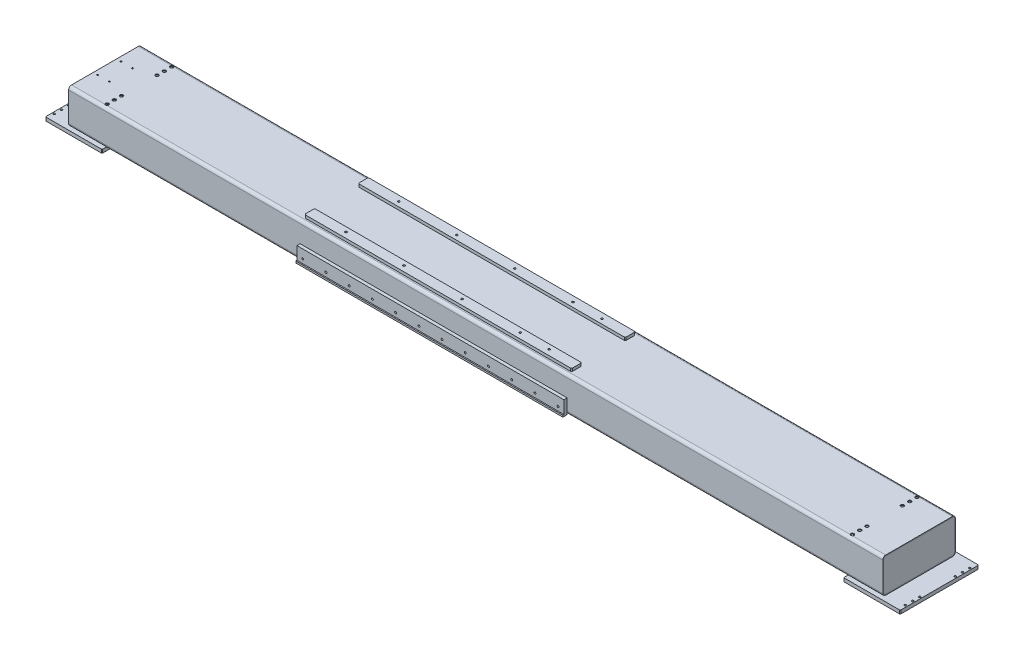
from build123d import *

# Parameters (mm, degrees)
F_250_X_120_X_3_0_1_DEPTH      = 2805
EXTRUDE_1_DEPTH                = 5
EXTRUDE_2_DEPTH                = 12
EXTRUDE_2_2_DEPTH              = 12
SKETCH_9_W                     = 920
SKETCH_9_H                     = 35
EXTRUDE_3_DEPTH                = 10
EXTRUDE_3_2_DEPTH              = 10
HOLE_WIZARD_M8_1_AT_2_COUNT    = 2
HOLE_WIZARD_M8_1_AT_2_PITCH    = 182
HOLE_WIZARD_M8_1_AT_3_COUNT    = 2
HOLE_WIZARD_M8_1_AT_3_PITCH    = 200
HOLE_WIZARD_M8_1_AT_4_COUNT    = 2
HOLE_WIZARD_M8_1_AT_4_PITCH    = 270.414496653
HOLE_WIZARD_M8_1_AT_5_COUNT    = 2
HOLE_WIZARD_M8_1_AT_5_PITCH    = 400
HOLE_WIZARD_M8_1_AT_6_COUNT    = 2
HOLE_WIZARD_M8_1_AT_6_PITCH    = 439.458758019
HOLE_WIZARD_M8_1_AT_7_COUNT    = 2
HOLE_WIZARD_M8_1_AT_7_PITCH    = 600
HOLE_WIZARD_M8_1_AT_8_COUNT    = 2
HOLE_WIZARD_M8_1_AT_8_PITCH    = 626.996012746
HOLE_WIZARD_M8_1_AT_9_COUNT    = 2
HOLE_WIZARD_M8_1_AT_9_PITCH    = 723.273115773
HOLE_WIZARD_M8_1_AT_10_COUNT   = 2
HOLE_WIZARD_M8_1_AT_10_PITCH   = 700
SKETCH_12_W                    = 920
SKETCH_12_H                    = 50
EXTRUDE_4_DEPTH                = 15
HOLE_WIZARD_M6_1_AT_2_COUNT    = 2
HOLE_WIZARD_M6_1_AT_2_PITCH    = 450
HOLE_WIZARD_M6_1_AT_3_COUNT    = 2
HOLE_WIZARD_M6_1_AT_3_PITCH    = 900
HOLE_WIZARD_M6_2_AT_2_COUNT    = 2
HOLE_WIZARD_M6_2_AT_2_PITCH    = 80
HOLE_WIZARD_M6_2_AT_3_COUNT    = 2
HOLE_WIZARD_M6_2_AT_3_PITCH    = 40
HOLE_WIZARD_M6_2_AT_4_COUNT    = 2
HOLE_WIZARD_M6_2_AT_4_PITCH    = 89.4427191
CHAMFER_1_SIZE                 = 3
CHAMFER_2_SIZE                 = 3
SKETCH_22_W                    = 3.3
SKETCH_22_H                    = 12
HOLE_WIZARD_M6_1_2_AT_2_COUNT  = 2
HOLE_WIZARD_M6_1_2_AT_2_PITCH  = 182
HOLE_WIZARD_M6_1_2_AT_3_COUNT  = 2
HOLE_WIZARD_M6_1_2_AT_3_PITCH  = 219.10727966
HOLE_WIZARD_M6_1_2_AT_4_COUNT  = 2
HOLE_WIZARD_M6_1_2_AT_4_PITCH  = 122
HOLE_WIZARD_M6_1_2_AT_5_COUNT  = 2
HOLE_WIZARD_M6_1_2_AT_5_PITCH  = 147
HOLE_WIZARD_M6_1_2_AT_6_COUNT  = 2
HOLE_WIZARD_M6_1_2_AT_6_PITCH  = 172
HOLE_WIZARD_M6_1_2_AT_7_COUNT  = 2
HOLE_WIZARD_M6_1_2_AT_7_PITCH  = 250.415654463
HOLE_WIZARD_M6_1_2_AT_8_COUNT  = 2
HOLE_WIZARD_M6_1_2_AT_8_PITCH  = 233.950849539
HOLE_WIZARD_M6_1_2_AT_9_COUNT  = 2
HOLE_WIZARD_M6_1_2_AT_9_PITCH  = 183.709009033
HOLE_WIZARD_M6_1_2_AT_10_COUNT = 2
HOLE_WIZARD_M6_1_2_AT_10_PITCH = 188.743211798
HOLE_WIZARD_M6_1_2_AT_11_COUNT = 2
HOLE_WIZARD_M6_1_2_AT_11_PITCH = 50
HOLE_WIZARD_M6_1_2_AT_12_COUNT = 2
HOLE_WIZARD_M6_1_2_AT_12_PITCH = 25
HOLE_WIZARD_M6_1_2_AT_13_COUNT = 2
HOLE_WIZARD_M6_1_2_AT_13_PITCH = 2932.1065806
HOLE_WIZARD_M6_1_2_AT_14_COUNT = 2
HOLE_WIZARD_M6_1_2_AT_14_PITCH = 2932.426299159
HOLE_WIZARD_M6_1_2_AT_15_COUNT = 2
HOLE_WIZARD_M6_1_2_AT_15_PITCH = 2750.454507895
HOLE_WIZARD_M6_1_2_AT_16_COUNT = 2
HOLE_WIZARD_M6_1_2_AT_16_PITCH = 2750.113634016
HOLE_WIZARD_M6_1_2_AT_17_COUNT = 2
HOLE_WIZARD_M6_1_2_AT_17_PITCH = 2750
HOLE_WIZARD_M6_1_2_AT_18_COUNT = 2
HOLE_WIZARD_M6_1_2_AT_18_PITCH = 2932
HOLE_WIZARD_M6_1_2_AT_19_COUNT = 2
HOLE_WIZARD_M6_1_2_AT_19_PITCH = 2753.926106489
HOLE_WIZARD_M6_1_2_AT_20_COUNT = 2
HOLE_WIZARD_M6_1_2_AT_20_PITCH = 2755.373658871
HOLE_WIZARD_M6_1_2_AT_21_COUNT = 2
HOLE_WIZARD_M6_1_2_AT_21_PITCH = 2937.040687495
HOLE_WIZARD_M6_1_2_AT_22_COUNT = 2
HOLE_WIZARD_M6_1_2_AT_22_PITCH = 2935.682714464
HOLE_WIZARD_M6_1_2_AT_23_COUNT = 2
HOLE_WIZARD_M6_1_2_AT_23_PITCH = 2934.537101486
HOLE_WIZARD_M6_1_2_AT_24_COUNT = 2
HOLE_WIZARD_M6_1_2_AT_24_PITCH = 2752.704851596
HOLE_WIZARD_1_AT_2_COUNT       = 2
HOLE_WIZARD_1_AT_2_PITCH       = 2568
HOLE_WIZARD_1_AT_3_COUNT       = 2
HOLE_WIZARD_1_AT_3_PITCH       = 2570.896341745
HOLE_WIZARD_1_AT_4_COUNT       = 2
HOLE_WIZARD_1_AT_4_PITCH       = 2568.121687148
HOLE_WIZARD_1_AT_5_COUNT       = 2
HOLE_WIZARD_1_AT_5_PITCH       = 2568.486714001
HOLE_WIZARD_1_AT_6_COUNT       = 2
HOLE_WIZARD_1_AT_6_PITCH       = 2572.203918821
HOLE_WIZARD_1_AT_7_COUNT       = 2
HOLE_WIZARD_1_AT_7_PITCH       = 2573.753678968
HOLE_WIZARD_1_AT_8_COUNT       = 2
HOLE_WIZARD_1_AT_8_PITCH       = 172
HOLE_WIZARD_1_AT_9_COUNT       = 2
HOLE_WIZARD_1_AT_9_PITCH       = 147
HOLE_WIZARD_1_AT_10_COUNT      = 2
HOLE_WIZARD_1_AT_10_PITCH      = 50
HOLE_WIZARD_1_AT_11_COUNT      = 2
HOLE_WIZARD_1_AT_11_PITCH      = 25
HOLE_WIZARD_1_AT_12_COUNT      = 2
HOLE_WIZARD_1_AT_12_PITCH      = 122
SKETCH_26_W                    = 920
SKETCH_26_H                    = 44
CUT_EXTRUDE_1_DEPTH            = 4
HOLE_WIZARD_M8_2_AT_2_COUNT    = 2
HOLE_WIZARD_M8_2_AT_2_PITCH    = 80
HOLE_WIZARD_M8_2_AT_3_COUNT    = 2
HOLE_WIZARD_M8_2_AT_3_PITCH    = 160
HOLE_WIZARD_M8_2_AT_4_COUNT    = 2
HOLE_WIZARD_M8_2_AT_4_PITCH    = 240
HOLE_WIZARD_M8_2_AT_5_COUNT    = 2
HOLE_WIZARD_M8_2_AT_5_PITCH    = 320
HOLE_WIZARD_M8_2_AT_6_COUNT    = 2
HOLE_WIZARD_M8_2_AT_6_PITCH    = 400
HOLE_WIZARD_M8_2_AT_7_COUNT    = 2
HOLE_WIZARD_M8_2_AT_7_PITCH    = 480
HOLE_WIZARD_M8_2_AT_8_COUNT    = 2
HOLE_WIZARD_M8_2_AT_8_PITCH    = 560
HOLE_WIZARD_M8_2_AT_9_COUNT    = 2
HOLE_WIZARD_M8_2_AT_9_PITCH    = 640
HOLE_WIZARD_M8_2_AT_10_COUNT   = 2
HOLE_WIZARD_M8_2_AT_10_PITCH   = 720
HOLE_WIZARD_M8_2_AT_11_COUNT   = 2
HOLE_WIZARD_M8_2_AT_11_PITCH   = 800
HOLE_WIZARD_M8_2_AT_12_COUNT   = 2
HOLE_WIZARD_M8_2_AT_12_PITCH   = 880


with BuildPart() as part:
    # Sketch11 → 矩型管 250 X 120 X 3.0(1) (new body)
    with BuildSketch(Plane.YZ.offset(-1402.5)):
        with BuildLine():
            Line((-50, -125), (50, -125))
            ThreePointArc((50, -125), (57.071067812, -122.071067812), (60, -115))
            Line((60, -115), (60, 115))
            ThreePointArc((60, 115), (57.071067812, 122.071067812), (50, 125))
            Line((50, 125), (-50, 125))
            ThreePointArc((-50, 125), (-57.071067812, 122.071067812), (-60, 115))
            Line((-60, 115), (-60, -115))
            ThreePointArc((-60, -115), (-57.071067812, -122.071067812), (-50, -125))
        make_face()
        with BuildLine():
            Line((-50, -122), (50, -122))
            ThreePointArc((50, -122), (54.949747468, -119.949747468), (57, -115))
            Line((57, -115), (57, 115))
            ThreePointArc((57, 115), (54.949747468, 119.949747468), (50, 122))
            Line((50, 122), (-50, 122))
            ThreePointArc((-50, 122), (-54.949747468, 119.949747468), (-57, 115))
            Line((-57, 115), (-57, -115))
            ThreePointArc((-57, -115), (-54.949747468, -119.949747468), (-50, -122))
        make_face(mode=Mode.SUBTRACT)
    extrude(amount=F_250_X_120_X_3_0_1_DEPTH)


with BuildPart() as body_2:
    # 草图3 → 凸台-拉伸1 (new body)
    with BuildSketch(Plane.ZY.offset(1402.5)):
        with BuildLine():
            Line((-122, -50), (-122, 50))
            ThreePointArc((-122, 50), (-119.949747468, 54.949747468), (-115, 57))
            Line((-115, 57), (115, 57))
            ThreePointArc((115, 57), (119.949747468, 54.949747468), (122, 50))
            Line((122, 50), (122, -50))
            ThreePointArc((122, -50), (119.949747468, -54.949747468), (115, -57))
            Line((115, -57), (-115, -57))
            ThreePointArc((-115, -57), (-119.949747468, -54.949747468), (-122, -50))
        make_face()
    extrude(amount=-EXTRUDE_1_DEPTH)


with BuildPart() as body_3:
    # 镜向1: mirrored copy
    add(body_2.part.mirror(Plane.XY))


with BuildPart() as body_4:
    # 镜向2: mirrored copy
    add(body_2.part.mirror(Plane(origin=(0, 0, 0), x_dir=(0, 0, 1), z_dir=(1, 0, 0))))


with BuildPart() as body_5:
    # Mirror 2 2: mirrored copy
    add(body_3.part.mirror(Plane(origin=(0, 0, 0), x_dir=(0, 0, 1), z_dir=(1, 0, 0))))


with BuildPart() as body_6:
    # 草图5 → 凸台-拉伸2 (new body)
    with BuildSketch(Plane(origin=(0, -60, -185), x_dir=(1, 0, 0), z_dir=(0, -1, 0))):
        Polygon((-1470.5, 320), (-1279.5, 320), (-1277.5, 318), (-1277.5, 52), (-1279.5, 50), (-1470.5, 50), (-1472.5, 52), (-1472.5, 318), align=None)
    extrude(amount=EXTRUDE_2_DEPTH)

    # 草图22 → Hole Wizard M6 _1 2 (revolve, cut)
    with BuildSketch(Plane(origin=(-1466, -60, -61), x_dir=(0, 0, 1), z_dir=(1, 0, 0))):
        with Locations((1.65, 6)):
            Rectangle(SKETCH_22_W, SKETCH_22_H)
    hole_wizard_m6_1_2 = revolve(axis=Axis((-1466, -53.65, -61), (0, -1, 0)), mode=Mode.SUBTRACT)

    # Hole Wizard M6 _1 2 at 2: Hole Wizard M6 _1 2 ×2
    with Locations(*[(i * HOLE_WIZARD_M6_1_2_AT_2_PITCH, 0, 0) for i in range(1, HOLE_WIZARD_M6_1_2_AT_2_COUNT)]):
        add(hole_wizard_m6_1_2, mode=Mode.SUBTRACT)

    # Hole Wizard M6 _1 2 at 3: Hole Wizard M6 _1 2 ×2
    with Locations(*[Vector(0.8306433281560934, -1.9052030489669335e-15, 0.5568048683244143) * (i * HOLE_WIZARD_M6_1_2_AT_3_PITCH) for i in range(1, HOLE_WIZARD_M6_1_2_AT_3_COUNT)]):
        add(hole_wizard_m6_1_2, mode=Mode.SUBTRACT)

    # Hole Wizard M6 _1 2 at 4: Hole Wizard M6 _1 2 ×2
    with Locations(*[(0, 0, i * HOLE_WIZARD_M6_1_2_AT_4_PITCH) for i in range(1, HOLE_WIZARD_M6_1_2_AT_4_COUNT)]):
        add(hole_wizard_m6_1_2, mode=Mode.SUBTRACT)

    # Hole Wizard M6 _1 2 at 5: Hole Wizard M6 _1 2 ×2
    with Locations(*[(0, 0, i * HOLE_WIZARD_M6_1_2_AT_5_PITCH) for i in range(1, HOLE_WIZARD_M6_1_2_AT_5_COUNT)]):
        add(hole_wizard_m6_1_2, mode=Mode.SUBTRACT)

    # Hole Wizard M6 _1 2 at 6: Hole Wizard M6 _1 2 ×2
    with Locations(*[(0, 0, i * HOLE_WIZARD_M6_1_2_AT_6_PITCH) for i in range(1, HOLE_WIZARD_M6_1_2_AT_6_COUNT)]):
        add(hole_wizard_m6_1_2, mode=Mode.SUBTRACT)

    # Hole Wizard M6 _1 2 at 7: Hole Wizard M6 _1 2 ×2
    with Locations(*[Vector(0.7267916232732317, -2.3479926408873147e-15, 0.6868580175988783) * (i * HOLE_WIZARD_M6_1_2_AT_7_PITCH) for i in range(1, HOLE_WIZARD_M6_1_2_AT_7_COUNT)]):
        add(hole_wizard_m6_1_2, mode=Mode.SUBTRACT)

    # Hole Wizard M6 _1 2 at 8: Hole Wizard M6 _1 2 ×2
    with Locations(*[Vector(0.7779411802037216, -2.1487803380109524e-15, 0.6283371070876212) * (i * HOLE_WIZARD_M6_1_2_AT_8_PITCH) for i in range(1, HOLE_WIZARD_M6_1_2_AT_8_COUNT)]):
        add(hole_wizard_m6_1_2, mode=Mode.SUBTRACT)

    # Hole Wizard M6 _1 2 at 9: Hole Wizard M6 _1 2 ×2
    with Locations(*[Vector(0.9906971952965136, 0, -0.1360847795736969) * (i * HOLE_WIZARD_M6_1_2_AT_9_PITCH) for i in range(1, HOLE_WIZARD_M6_1_2_AT_9_COUNT)]):
        add(hole_wizard_m6_1_2, mode=Mode.SUBTRACT)

    # Hole Wizard M6 _1 2 at 10: Hole Wizard M6 _1 2 ×2
    with Locations(*[Vector(0.9642730896957256, 0, -0.2649101894768476) * (i * HOLE_WIZARD_M6_1_2_AT_10_PITCH) for i in range(1, HOLE_WIZARD_M6_1_2_AT_10_COUNT)]):
        add(hole_wizard_m6_1_2, mode=Mode.SUBTRACT)

    # Hole Wizard M6 _1 2 at 11: Hole Wizard M6 _1 2 ×2
    with Locations(*[(0, 0, -i * HOLE_WIZARD_M6_1_2_AT_11_PITCH) for i in range(1, HOLE_WIZARD_M6_1_2_AT_11_COUNT)]):
        add(hole_wizard_m6_1_2, mode=Mode.SUBTRACT)

    # Hole Wizard M6 _1 2 at 12: Hole Wizard M6 _1 2 ×2
    with Locations(*[(0, 0, -i * HOLE_WIZARD_M6_1_2_AT_12_PITCH) for i in range(1, HOLE_WIZARD_M6_1_2_AT_12_COUNT)]):
        add(hole_wizard_m6_1_2, mode=Mode.SUBTRACT)


with BuildPart() as body_7:
    # 草图5 → Extrude 2 2 (new body)
    with BuildSketch(Plane(origin=(0, -60, -185), x_dir=(1, 0, 0), z_dir=(0, -1, 0))):
        Polygon((1472.5, 318), (1470.5, 320), (1279.5, 320), (1277.5, 318), (1277.5, 52), (1279.5, 50), (1470.5, 50), (1472.5, 52), align=None)
    extrude(amount=EXTRUDE_2_2_DEPTH)

    # Hole Wizard M6 _1 2 at 13: Hole Wizard M6 _1 2 ×2
    with Locations(*[Vector(0.9999636505026536, 0, -0.008526293063631086) * (i * HOLE_WIZARD_M6_1_2_AT_13_PITCH) for i in range(1, HOLE_WIZARD_M6_1_2_AT_13_COUNT)]):
        add(hole_wizard_m6_1_2, mode=Mode.SUBTRACT)

    # Hole Wizard M6 _1 2 at 14: Hole Wizard M6 _1 2 ×2
    with Locations(*[Vector(0.9998546257891517, 0, -0.01705072690636343) * (i * HOLE_WIZARD_M6_1_2_AT_14_PITCH) for i in range(1, HOLE_WIZARD_M6_1_2_AT_14_COUNT)]):
        add(hole_wizard_m6_1_2, mode=Mode.SUBTRACT)

    # Hole Wizard M6 _1 2 at 15: Hole Wizard M6 _1 2 ×2
    with Locations(*[Vector(0.9998347517133228, 0, -0.018178813667514955) * (i * HOLE_WIZARD_M6_1_2_AT_15_PITCH) for i in range(1, HOLE_WIZARD_M6_1_2_AT_15_COUNT)]):
        add(hole_wizard_m6_1_2, mode=Mode.SUBTRACT)

    # Hole Wizard M6 _1 2 at 16: Hole Wizard M6 _1 2 ×2
    with Locations(*[Vector(0.9999586802470746, 0, -0.009090533456791589) * (i * HOLE_WIZARD_M6_1_2_AT_16_PITCH) for i in range(1, HOLE_WIZARD_M6_1_2_AT_16_COUNT)]):
        add(hole_wizard_m6_1_2, mode=Mode.SUBTRACT)

    # Hole Wizard M6 _1 2 at 17: Hole Wizard M6 _1 2 ×2
    with Locations(*[(i * HOLE_WIZARD_M6_1_2_AT_17_PITCH, 0, 0) for i in range(1, HOLE_WIZARD_M6_1_2_AT_17_COUNT)]):
        add(hole_wizard_m6_1_2, mode=Mode.SUBTRACT)

    # Hole Wizard M6 _1 2 at 18: Hole Wizard M6 _1 2 ×2
    with Locations(*[(i * HOLE_WIZARD_M6_1_2_AT_18_PITCH, 0, 0) for i in range(1, HOLE_WIZARD_M6_1_2_AT_18_COUNT)]):
        add(hole_wizard_m6_1_2, mode=Mode.SUBTRACT)

    # Hole Wizard M6 _1 2 at 19: Hole Wizard M6 _1 2 ×2
    with Locations(*[Vector(0.9985743602635353, 0, 0.05337833853045079) * (i * HOLE_WIZARD_M6_1_2_AT_19_PITCH) for i in range(1, HOLE_WIZARD_M6_1_2_AT_19_COUNT)]):
        add(hole_wizard_m6_1_2, mode=Mode.SUBTRACT)

    # Hole Wizard M6 _1 2 at 20: Hole Wizard M6 _1 2 ×2
    with Locations(*[Vector(0.9980497531238023, 0, 0.062423475468106907) * (i * HOLE_WIZARD_M6_1_2_AT_20_PITCH) for i in range(1, HOLE_WIZARD_M6_1_2_AT_20_COUNT)]):
        add(hole_wizard_m6_1_2, mode=Mode.SUBTRACT)

    # Hole Wizard M6 _1 2 at 21: Hole Wizard M6 _1 2 ×2
    with Locations(*[Vector(0.9982837529230445, 0, 0.05856234839794122) * (i * HOLE_WIZARD_M6_1_2_AT_21_PITCH) for i in range(1, HOLE_WIZARD_M6_1_2_AT_21_COUNT)]):
        add(hole_wizard_m6_1_2, mode=Mode.SUBTRACT)

    # Hole Wizard M6 _1 2 at 22: Hole Wizard M6 _1 2 ×2
    with Locations(*[Vector(0.9987455338939073, 0, 0.05007353120136575) * (i * HOLE_WIZARD_M6_1_2_AT_22_PITCH) for i in range(1, HOLE_WIZARD_M6_1_2_AT_22_COUNT)]):
        add(hole_wizard_m6_1_2, mode=Mode.SUBTRACT)

    # Hole Wizard M6 _1 2 at 23: Hole Wizard M6 _1 2 ×2
    with Locations(*[Vector(0.9991354338355168, 0, 0.04157384820188713) * (i * HOLE_WIZARD_M6_1_2_AT_23_PITCH) for i in range(1, HOLE_WIZARD_M6_1_2_AT_23_COUNT)]):
        add(hole_wizard_m6_1_2, mode=Mode.SUBTRACT)

    # Hole Wizard M6 _1 2 at 24: Hole Wizard M6 _1 2 ×2
    with Locations(*[Vector(0.9990173840851833, 0, 0.04432004394850631) * (i * HOLE_WIZARD_M6_1_2_AT_24_PITCH) for i in range(1, HOLE_WIZARD_M6_1_2_AT_24_COUNT)]):
        add(hole_wizard_m6_1_2, mode=Mode.SUBTRACT)


with BuildPart() as body_8:
    # 草图9 → 凸台-拉伸3 (new body)
    with BuildSketch(Plane(origin=(0, 60, 0), x_dir=(1, 0, 0), z_dir=(0, 1, 0))):
        with Locations((-145, 92.5)):
            Rectangle(SKETCH_9_W, SKETCH_9_H)
    extrude(amount=EXTRUDE_3_DEPTH)


with BuildPart() as body_9:
    # 草图9 → Extrude 3 2 (new body)
    with BuildSketch(Plane(origin=(0, 60, 0), x_dir=(1, 0, 0), z_dir=(0, 1, 0))):
        with Locations((-145, -92.5)):
            Rectangle(SKETCH_9_W, SKETCH_9_H)
    extrude(amount=EXTRUDE_3_2_DEPTH)


with BuildPart() as hole_wizard_m8_1_tool:
    # 草图11 → Hole Wizard M8 _1 (revolve)
    with BuildSketch(Plane(origin=(-481, 70, -91), x_dir=(0, 0, 1), z_dir=(1, 0, 0))):
        Polygon((0, 0), (0, 21.792926105), (3.4, 19.75), (3.4, 0), align=None)
    hole_wizard_m8_1 = revolve(axis=Axis((-481, 76.35, -91), (0, -1, 0)))


with BuildPart() as part_1:
    add(part.part)

    # Hole Wizard M8 _1: cut by hole_wizard_m8_1_tool
    add(hole_wizard_m8_1_tool.part, mode=Mode.SUBTRACT)


with BuildPart() as body_8_1:
    add(body_8.part)

    # Hole Wizard M8 _1: cut by hole_wizard_m8_1_tool
    add(hole_wizard_m8_1_tool.part, mode=Mode.SUBTRACT)


with BuildPart() as hole_wizard_m8_1_at_2_tool:
    # Hole Wizard M8 _1 at 2: Hole Wizard M8 _1 ×2
    with Locations(*[(0, 0, i * HOLE_WIZARD_M8_1_AT_2_PITCH) for i in range(1, HOLE_WIZARD_M8_1_AT_2_COUNT)]):
        add(hole_wizard_m8_1)


with BuildPart() as part_2:
    add(part_1.part)

    # Hole Wizard M8 _1 at 2: cut by hole_wizard_m8_1_at_2_tool
    add(hole_wizard_m8_1_at_2_tool.part, mode=Mode.SUBTRACT)


with BuildPart() as body_9_1:
    add(body_9.part)

    # Hole Wizard M8 _1 at 2: cut by hole_wizard_m8_1_at_2_tool
    add(hole_wizard_m8_1_at_2_tool.part, mode=Mode.SUBTRACT)


with BuildPart() as hole_wizard_m8_1_at_3_tool:
    # Hole Wizard M8 _1 at 3: Hole Wizard M8 _1 ×2
    with Locations(*[(i * HOLE_WIZARD_M8_1_AT_3_PITCH, 0, 0) for i in range(1, HOLE_WIZARD_M8_1_AT_3_COUNT)]):
        add(hole_wizard_m8_1)


with BuildPart() as part_3:
    add(part_2.part)

    # Hole Wizard M8 _1 at 3: cut by hole_wizard_m8_1_at_3_tool
    add(hole_wizard_m8_1_at_3_tool.part, mode=Mode.SUBTRACT)


with BuildPart() as body_8_2:
    add(body_8_1.part)

    # Hole Wizard M8 _1 at 3: cut by hole_wizard_m8_1_at_3_tool
    add(hole_wizard_m8_1_at_3_tool.part, mode=Mode.SUBTRACT)


with BuildPart() as hole_wizard_m8_1_at_4_tool:
    # Hole Wizard M8 _1 at 4: Hole Wizard M8 _1 ×2
    with Locations(*[Vector(0.7396053187813598, 0, 0.6730408400909437) * (i * HOLE_WIZARD_M8_1_AT_4_PITCH) for i in range(1, HOLE_WIZARD_M8_1_AT_4_COUNT)]):
        add(hole_wizard_m8_1)


with BuildPart() as part_4:
    add(part_3.part)

    # Hole Wizard M8 _1 at 4: cut by hole_wizard_m8_1_at_4_tool
    add(hole_wizard_m8_1_at_4_tool.part, mode=Mode.SUBTRACT)


with BuildPart() as body_9_2:
    add(body_9_1.part)

    # Hole Wizard M8 _1 at 4: cut by hole_wizard_m8_1_at_4_tool
    add(hole_wizard_m8_1_at_4_tool.part, mode=Mode.SUBTRACT)


with BuildPart() as hole_wizard_m8_1_at_5_tool:
    # Hole Wizard M8 _1 at 5: Hole Wizard M8 _1 ×2
    with Locations(*[(i * HOLE_WIZARD_M8_1_AT_5_PITCH, 0, 0) for i in range(1, HOLE_WIZARD_M8_1_AT_5_COUNT)]):
        add(hole_wizard_m8_1)


with BuildPart() as part_5:
    add(part_4.part)

    # Hole Wizard M8 _1 at 5: cut by hole_wizard_m8_1_at_5_tool
    add(hole_wizard_m8_1_at_5_tool.part, mode=Mode.SUBTRACT)


with BuildPart() as body_8_3:
    add(body_8_2.part)

    # Hole Wizard M8 _1 at 5: cut by hole_wizard_m8_1_at_5_tool
    add(hole_wizard_m8_1_at_5_tool.part, mode=Mode.SUBTRACT)


with BuildPart() as hole_wizard_m8_1_at_6_tool:
    # Hole Wizard M8 _1 at 6: Hole Wizard M8 _1 ×2
    with Locations(*[Vector(0.9102105549169733, 0, 0.4141458024871621) * (i * HOLE_WIZARD_M8_1_AT_6_PITCH) for i in range(1, HOLE_WIZARD_M8_1_AT_6_COUNT)]):
        add(hole_wizard_m8_1)


with BuildPart() as part_6:
    add(part_5.part)

    # Hole Wizard M8 _1 at 6: cut by hole_wizard_m8_1_at_6_tool
    add(hole_wizard_m8_1_at_6_tool.part, mode=Mode.SUBTRACT)


with BuildPart() as body_9_3:
    add(body_9_2.part)

    # Hole Wizard M8 _1 at 6: cut by hole_wizard_m8_1_at_6_tool
    add(hole_wizard_m8_1_at_6_tool.part, mode=Mode.SUBTRACT)


with BuildPart() as hole_wizard_m8_1_at_7_tool:
    # Hole Wizard M8 _1 at 7: Hole Wizard M8 _1 ×2
    with Locations(*[(i * HOLE_WIZARD_M8_1_AT_7_PITCH, 0, 0) for i in range(1, HOLE_WIZARD_M8_1_AT_7_COUNT)]):
        add(hole_wizard_m8_1)


with BuildPart() as part_7:
    add(part_6.part)

    # Hole Wizard M8 _1 at 7: cut by hole_wizard_m8_1_at_7_tool
    add(hole_wizard_m8_1_at_7_tool.part, mode=Mode.SUBTRACT)


with BuildPart() as body_8_4:
    add(body_8_3.part)

    # Hole Wizard M8 _1 at 7: cut by hole_wizard_m8_1_at_7_tool
    add(hole_wizard_m8_1_at_7_tool.part, mode=Mode.SUBTRACT)


with BuildPart() as hole_wizard_m8_1_at_8_tool:
    # Hole Wizard M8 _1 at 8: Hole Wizard M8 _1 ×2
    with Locations(*[Vector(0.9569438844942066, 0, 0.2902729782965312) * (i * HOLE_WIZARD_M8_1_AT_8_PITCH) for i in range(1, HOLE_WIZARD_M8_1_AT_8_COUNT)]):
        add(hole_wizard_m8_1)


with BuildPart() as part_8:
    add(part_7.part)

    # Hole Wizard M8 _1 at 8: cut by hole_wizard_m8_1_at_8_tool
    add(hole_wizard_m8_1_at_8_tool.part, mode=Mode.SUBTRACT)


with BuildPart() as body_9_4:
    add(body_9_3.part)

    # Hole Wizard M8 _1 at 8: cut by hole_wizard_m8_1_at_8_tool
    add(hole_wizard_m8_1_at_8_tool.part, mode=Mode.SUBTRACT)


with BuildPart() as hole_wizard_m8_1_at_9_tool:
    # Hole Wizard M8 _1 at 9: Hole Wizard M8 _1 ×2
    with Locations(*[Vector(0.9678225067882815, 0, 0.2516338517649143) * (i * HOLE_WIZARD_M8_1_AT_9_PITCH) for i in range(1, HOLE_WIZARD_M8_1_AT_9_COUNT)]):
        add(hole_wizard_m8_1)


with BuildPart() as part_9:
    add(part_8.part)

    # Hole Wizard M8 _1 at 9: cut by hole_wizard_m8_1_at_9_tool
    add(hole_wizard_m8_1_at_9_tool.part, mode=Mode.SUBTRACT)


with BuildPart() as body_9_5:
    add(body_9_4.part)

    # Hole Wizard M8 _1 at 9: cut by hole_wizard_m8_1_at_9_tool
    add(hole_wizard_m8_1_at_9_tool.part, mode=Mode.SUBTRACT)

    # 倒角2
    chamfer_2_edges = [body_9_5.edges().sort_by_distance(p)[0] for p in [
        (-605, 65, 110),
        (-605, 65, 75),
        (315, 65, 75),
        (315, 65, 110),
    ]]
    chamfer(chamfer_2_edges, length=CHAMFER_2_SIZE)


with BuildPart() as hole_wizard_m8_1_at_10_tool:
    # Hole Wizard M8 _1 at 10: Hole Wizard M8 _1 ×2
    with Locations(*[(i * HOLE_WIZARD_M8_1_AT_10_PITCH, 0, 0) for i in range(1, HOLE_WIZARD_M8_1_AT_10_COUNT)]):
        add(hole_wizard_m8_1)


with BuildPart() as part_10:
    add(part_9.part)

    # Hole Wizard M8 _1 at 10: cut by hole_wizard_m8_1_at_10_tool
    add(hole_wizard_m8_1_at_10_tool.part, mode=Mode.SUBTRACT)

    # 草图18 → Hole Wizard M6 _1 (revolve, cut)
    with BuildSketch(Plane(origin=(305, -15, -125), x_dir=(0, 1, 0), z_dir=(1, 0, 0))):
        Polygon((0, 0), (0, 16.502151548), (2.5, 15), (2.5, 0), align=None)
    hole_wizard_m6_1 = revolve(axis=Axis((305, -15, -131.35), (0, 0, 1)), mode=Mode.SUBTRACT)

    # Hole Wizard M6 _1 at 2: Hole Wizard M6 _1 ×2
    with Locations(*[(-i * HOLE_WIZARD_M6_1_AT_2_PITCH, 0, 0) for i in range(1, HOLE_WIZARD_M6_1_AT_2_COUNT)]):
        add(hole_wizard_m6_1, mode=Mode.SUBTRACT)

    # Hole Wizard M6 _1 at 3: Hole Wizard M6 _1 ×2
    with Locations(*[(-i * HOLE_WIZARD_M6_1_AT_3_PITCH, 0, 0) for i in range(1, HOLE_WIZARD_M6_1_AT_3_COUNT)]):
        add(hole_wizard_m6_1, mode=Mode.SUBTRACT)

    # 草图20 → M6 螺纹孔2 (revolve, cut)
    with BuildSketch(Plane(origin=(-1387.5, 60, 40), x_dir=(0, 0, 1), z_dir=(1, 0, 0))):
        Polygon((0, 0), (0, 16.502151548), (2.5, 15), (2.5, 0), align=None)
    hole_wizard_m6_2 = revolve(axis=Axis((-1387.5, 66.35, 40), (0, -1, 0)), mode=Mode.SUBTRACT)

    # M6 螺纹孔2 at 2: M6 螺纹孔2 ×2
    with Locations(*[(0, 0, -i * HOLE_WIZARD_M6_2_AT_2_PITCH) for i in range(1, HOLE_WIZARD_M6_2_AT_2_COUNT)]):
        add(hole_wizard_m6_2, mode=Mode.SUBTRACT)

    # M6 螺纹孔2 at 3: M6 螺纹孔2 ×2
    with Locations(*[(i * HOLE_WIZARD_M6_2_AT_3_PITCH, 0, 0) for i in range(1, HOLE_WIZARD_M6_2_AT_3_COUNT)]):
        add(hole_wizard_m6_2, mode=Mode.SUBTRACT)

    # M6 螺纹孔2 at 4: M6 螺纹孔2 ×2
    with Locations(*[Vector(0.447213595499958, 3.1180628964785753e-15, -0.894427190999916) * (i * HOLE_WIZARD_M6_2_AT_4_PITCH) for i in range(1, HOLE_WIZARD_M6_2_AT_4_COUNT)]):
        add(hole_wizard_m6_2, mode=Mode.SUBTRACT)

    # 草图25 → 打孔尺寸(%根据)内六角圆柱头螺钉的类型1 (revolve, cut)
    with BuildSketch(Plane(origin=(1284, 60, 61), x_dir=(0, 0, 1), z_dir=(1, 0, 0))):
        Polygon((0, 0), (0, 132), (3.3, 132), (3.3, 6.8), (5.5, 6.8), (5.5, 0), align=None)
    hole_wizard_1 = revolve(axis=Axis((1284, 66.35, 61), (0, -1, 0)), mode=Mode.SUBTRACT)

    # 打孔尺寸(%根据)内六角圆柱头螺钉的类型1 at 2: 打孔尺寸(%根据)内六角圆柱头螺钉的类型1 ×2
    with Locations(*[(-i * HOLE_WIZARD_1_AT_2_PITCH, 0, 0) for i in range(1, HOLE_WIZARD_1_AT_2_COUNT)]):
        add(hole_wizard_1, mode=Mode.SUBTRACT)

    # 打孔尺寸(%根据)内六角圆柱头螺钉的类型1 at 3: 打孔尺寸(%根据)内六角圆柱头螺钉的类型1 ×2
    with Locations(*[Vector(-0.9988734116975495, 0, -0.04745426644357505) * (i * HOLE_WIZARD_1_AT_3_PITCH) for i in range(1, HOLE_WIZARD_1_AT_3_COUNT)]):
        add(hole_wizard_1, mode=Mode.SUBTRACT)

    # 打孔尺寸(%根据)内六角圆柱头螺钉的类型1 at 4: 打孔尺寸(%根据)内六角圆柱头螺钉的类型1 ×2
    with Locations(*[Vector(-0.9999526162842554, 0, 0.009734741202144355) * (i * HOLE_WIZARD_1_AT_4_PITCH) for i in range(1, HOLE_WIZARD_1_AT_4_COUNT)]):
        add(hole_wizard_1, mode=Mode.SUBTRACT)

    # 打孔尺寸(%根据)内六角圆柱头螺钉的类型1 at 5: 打孔尺寸(%根据)内六角圆柱头螺钉的类型1 ×2
    with Locations(*[Vector(-0.9998105055407085, 0, 0.019466715450559086) * (i * HOLE_WIZARD_1_AT_5_PITCH) for i in range(1, HOLE_WIZARD_1_AT_5_COUNT)]):
        add(hole_wizard_1, mode=Mode.SUBTRACT)

    # 打孔尺寸(%根据)内六角圆柱头螺钉的类型1 at 6: 打孔尺寸(%根据)内六角圆柱头螺钉的类型1 ×2
    with Locations(*[Vector(-0.9983656354806839, 0, -0.05714943474130069) * (i * HOLE_WIZARD_1_AT_6_PITCH) for i in range(1, HOLE_WIZARD_1_AT_6_COUNT)]):
        add(hole_wizard_1, mode=Mode.SUBTRACT)

    # 打孔尺寸(%根据)内六角圆柱头螺钉的类型1 at 7: 打孔尺寸(%根据)内六角圆柱头螺钉的类型1 ×2
    with Locations(*[Vector(-0.99776447955577, 0, -0.06682846202632091) * (i * HOLE_WIZARD_1_AT_7_PITCH) for i in range(1, HOLE_WIZARD_1_AT_7_COUNT)]):
        add(hole_wizard_1, mode=Mode.SUBTRACT)

    # 打孔尺寸(%根据)内六角圆柱头螺钉的类型1 at 8: 打孔尺寸(%根据)内六角圆柱头螺钉的类型1 ×2
    with Locations(*[(0, 0, -i * HOLE_WIZARD_1_AT_8_PITCH) for i in range(1, HOLE_WIZARD_1_AT_8_COUNT)]):
        add(hole_wizard_1, mode=Mode.SUBTRACT)

    # 打孔尺寸(%根据)内六角圆柱头螺钉的类型1 at 9: 打孔尺寸(%根据)内六角圆柱头螺钉的类型1 ×2
    with Locations(*[(0, 0, -i * HOLE_WIZARD_1_AT_9_PITCH) for i in range(1, HOLE_WIZARD_1_AT_9_COUNT)]):
        add(hole_wizard_1, mode=Mode.SUBTRACT)

    # 打孔尺寸(%根据)内六角圆柱头螺钉的类型1 at 10: 打孔尺寸(%根据)内六角圆柱头螺钉的类型1 ×2
    with Locations(*[(0, 0, i * HOLE_WIZARD_1_AT_10_PITCH) for i in range(1, HOLE_WIZARD_1_AT_10_COUNT)]):
        add(hole_wizard_1, mode=Mode.SUBTRACT)

    # 打孔尺寸(%根据)内六角圆柱头螺钉的类型1 at 11: 打孔尺寸(%根据)内六角圆柱头螺钉的类型1 ×2
    with Locations(*[(0, 0, i * HOLE_WIZARD_1_AT_11_PITCH) for i in range(1, HOLE_WIZARD_1_AT_11_COUNT)]):
        add(hole_wizard_1, mode=Mode.SUBTRACT)

    # 打孔尺寸(%根据)内六角圆柱头螺钉的类型1 at 12: 打孔尺寸(%根据)内六角圆柱头螺钉的类型1 ×2
    with Locations(*[(0, 0, -i * HOLE_WIZARD_1_AT_12_PITCH) for i in range(1, HOLE_WIZARD_1_AT_12_COUNT)]):
        add(hole_wizard_1, mode=Mode.SUBTRACT)


with BuildPart() as body_8_5:
    add(body_8_4.part)

    # Hole Wizard M8 _1 at 10: cut by hole_wizard_m8_1_at_10_tool
    add(hole_wizard_m8_1_at_10_tool.part, mode=Mode.SUBTRACT)

    # 倒角1
    chamfer_1_edges = [body_8_5.edges().sort_by_distance(p)[0] for p in [
        (-605, 65, -110),
        (315, 65, -110),
        (315, 65, -75),
        (-605, 65, -75),
    ]]
    chamfer(chamfer_1_edges, length=CHAMFER_1_SIZE)


with BuildPart() as body_10:
    # 草图12 → 凸台-拉伸4 (new body)
    with BuildSketch(Plane(origin=(0, 65, 125), x_dir=(1, 0, 0), z_dir=(0, 0, -1))):
        with Locations((-145, 100)):
            Rectangle(SKETCH_12_W, SKETCH_12_H)
    extrude(amount=-EXTRUDE_4_DEPTH)

    # 草图26 → 切除-拉伸1 (cut)
    with BuildSketch(Plane.XY.offset(140)):
        with Locations((-145, -32)):
            Rectangle(SKETCH_26_W, SKETCH_26_H)
    extrude(amount=-CUT_EXTRUDE_1_DEPTH, mode=Mode.SUBTRACT)


with BuildPart() as hole_wizard_m8_2_tool:
    # 草图14 → M8 螺纹孔2 (revolve)
    with BuildSketch(Plane(origin=(-585, -40, 136), x_dir=(0, -1, 0), z_dir=(1, 0, 0))):
        Polygon((0, 0), (0, 21.792926105), (3.4, 19.75), (3.4, 0), align=None)
    hole_wizard_m8_2 = revolve(axis=Axis((-585, -40, 142.35), (0, 0, -1)))


with BuildPart() as part_11:
    add(part_10.part)

    # M8 螺纹孔2: cut by hole_wizard_m8_2_tool
    add(hole_wizard_m8_2_tool.part, mode=Mode.SUBTRACT)


with BuildPart() as body_10_1:
    add(body_10.part)

    # M8 螺纹孔2: cut by hole_wizard_m8_2_tool
    add(hole_wizard_m8_2_tool.part, mode=Mode.SUBTRACT)


with BuildPart() as hole_wizard_m8_2_at_2_tool:
    # M8 螺纹孔2 at 2: M8 螺纹孔2 ×2
    with Locations(*[(i * HOLE_WIZARD_M8_2_AT_2_PITCH, 0, 0) for i in range(1, HOLE_WIZARD_M8_2_AT_2_COUNT)]):
        add(hole_wizard_m8_2)


with BuildPart() as part_12:
    add(part_11.part)

    # M8 螺纹孔2 at 2: cut by hole_wizard_m8_2_at_2_tool
    add(hole_wizard_m8_2_at_2_tool.part, mode=Mode.SUBTRACT)


with BuildPart() as body_10_2:
    add(body_10_1.part)

    # M8 螺纹孔2 at 2: cut by hole_wizard_m8_2_at_2_tool
    add(hole_wizard_m8_2_at_2_tool.part, mode=Mode.SUBTRACT)


with BuildPart() as hole_wizard_m8_2_at_3_tool:
    # M8 螺纹孔2 at 3: M8 螺纹孔2 ×2
    with Locations(*[(i * HOLE_WIZARD_M8_2_AT_3_PITCH, 0, 0) for i in range(1, HOLE_WIZARD_M8_2_AT_3_COUNT)]):
        add(hole_wizard_m8_2)


with BuildPart() as part_13:
    add(part_12.part)

    # M8 螺纹孔2 at 3: cut by hole_wizard_m8_2_at_3_tool
    add(hole_wizard_m8_2_at_3_tool.part, mode=Mode.SUBTRACT)


with BuildPart() as body_10_3:
    add(body_10_2.part)

    # M8 螺纹孔2 at 3: cut by hole_wizard_m8_2_at_3_tool
    add(hole_wizard_m8_2_at_3_tool.part, mode=Mode.SUBTRACT)


with BuildPart() as hole_wizard_m8_2_at_4_tool:
    # M8 螺纹孔2 at 4: M8 螺纹孔2 ×2
    with Locations(*[(i * HOLE_WIZARD_M8_2_AT_4_PITCH, 0, 0) for i in range(1, HOLE_WIZARD_M8_2_AT_4_COUNT)]):
        add(hole_wizard_m8_2)


with BuildPart() as part_14:
    add(part_13.part)

    # M8 螺纹孔2 at 4: cut by hole_wizard_m8_2_at_4_tool
    add(hole_wizard_m8_2_at_4_tool.part, mode=Mode.SUBTRACT)


with BuildPart() as body_10_4:
    add(body_10_3.part)

    # M8 螺纹孔2 at 4: cut by hole_wizard_m8_2_at_4_tool
    add(hole_wizard_m8_2_at_4_tool.part, mode=Mode.SUBTRACT)


with BuildPart() as hole_wizard_m8_2_at_5_tool:
    # M8 螺纹孔2 at 5: M8 螺纹孔2 ×2
    with Locations(*[(i * HOLE_WIZARD_M8_2_AT_5_PITCH, 0, 0) for i in range(1, HOLE_WIZARD_M8_2_AT_5_COUNT)]):
        add(hole_wizard_m8_2)


with BuildPart() as part_15:
    add(part_14.part)

    # M8 螺纹孔2 at 5: cut by hole_wizard_m8_2_at_5_tool
    add(hole_wizard_m8_2_at_5_tool.part, mode=Mode.SUBTRACT)


with BuildPart() as body_10_5:
    add(body_10_4.part)

    # M8 螺纹孔2 at 5: cut by hole_wizard_m8_2_at_5_tool
    add(hole_wizard_m8_2_at_5_tool.part, mode=Mode.SUBTRACT)


with BuildPart() as hole_wizard_m8_2_at_6_tool:
    # M8 螺纹孔2 at 6: M8 螺纹孔2 ×2
    with Locations(*[(i * HOLE_WIZARD_M8_2_AT_6_PITCH, 0, 0) for i in range(1, HOLE_WIZARD_M8_2_AT_6_COUNT)]):
        add(hole_wizard_m8_2)


with BuildPart() as part_16:
    add(part_15.part)

    # M8 螺纹孔2 at 6: cut by hole_wizard_m8_2_at_6_tool
    add(hole_wizard_m8_2_at_6_tool.part, mode=Mode.SUBTRACT)


with BuildPart() as body_10_6:
    add(body_10_5.part)

    # M8 螺纹孔2 at 6: cut by hole_wizard_m8_2_at_6_tool
    add(hole_wizard_m8_2_at_6_tool.part, mode=Mode.SUBTRACT)


with BuildPart() as hole_wizard_m8_2_at_7_tool:
    # M8 螺纹孔2 at 7: M8 螺纹孔2 ×2
    with Locations(*[(i * HOLE_WIZARD_M8_2_AT_7_PITCH, 0, 0) for i in range(1, HOLE_WIZARD_M8_2_AT_7_COUNT)]):
        add(hole_wizard_m8_2)


with BuildPart() as part_17:
    add(part_16.part)

    # M8 螺纹孔2 at 7: cut by hole_wizard_m8_2_at_7_tool
    add(hole_wizard_m8_2_at_7_tool.part, mode=Mode.SUBTRACT)


with BuildPart() as body_10_7:
    add(body_10_6.part)

    # M8 螺纹孔2 at 7: cut by hole_wizard_m8_2_at_7_tool
    add(hole_wizard_m8_2_at_7_tool.part, mode=Mode.SUBTRACT)


with BuildPart() as hole_wizard_m8_2_at_8_tool:
    # M8 螺纹孔2 at 8: M8 螺纹孔2 ×2
    with Locations(*[(i * HOLE_WIZARD_M8_2_AT_8_PITCH, 0, 0) for i in range(1, HOLE_WIZARD_M8_2_AT_8_COUNT)]):
        add(hole_wizard_m8_2)


with BuildPart() as part_18:
    add(part_17.part)

    # M8 螺纹孔2 at 8: cut by hole_wizard_m8_2_at_8_tool
    add(hole_wizard_m8_2_at_8_tool.part, mode=Mode.SUBTRACT)


with BuildPart() as body_10_8:
    add(body_10_7.part)

    # M8 螺纹孔2 at 8: cut by hole_wizard_m8_2_at_8_tool
    add(hole_wizard_m8_2_at_8_tool.part, mode=Mode.SUBTRACT)


with BuildPart() as hole_wizard_m8_2_at_9_tool:
    # M8 螺纹孔2 at 9: M8 螺纹孔2 ×2
    with Locations(*[(i * HOLE_WIZARD_M8_2_AT_9_PITCH, 0, 0) for i in range(1, HOLE_WIZARD_M8_2_AT_9_COUNT)]):
        add(hole_wizard_m8_2)


with BuildPart() as part_19:
    add(part_18.part)

    # M8 螺纹孔2 at 9: cut by hole_wizard_m8_2_at_9_tool
    add(hole_wizard_m8_2_at_9_tool.part, mode=Mode.SUBTRACT)


with BuildPart() as body_10_9:
    add(body_10_8.part)

    # M8 螺纹孔2 at 9: cut by hole_wizard_m8_2_at_9_tool
    add(hole_wizard_m8_2_at_9_tool.part, mode=Mode.SUBTRACT)


with BuildPart() as hole_wizard_m8_2_at_10_tool:
    # M8 螺纹孔2 at 10: M8 螺纹孔2 ×2
    with Locations(*[(i * HOLE_WIZARD_M8_2_AT_10_PITCH, 0, 0) for i in range(1, HOLE_WIZARD_M8_2_AT_10_COUNT)]):
        add(hole_wizard_m8_2)


with BuildPart() as part_20:
    add(part_19.part)

    # M8 螺纹孔2 at 10: cut by hole_wizard_m8_2_at_10_tool
    add(hole_wizard_m8_2_at_10_tool.part, mode=Mode.SUBTRACT)


with BuildPart() as body_10_10:
    add(body_10_9.part)

    # M8 螺纹孔2 at 10: cut by hole_wizard_m8_2_at_10_tool
    add(hole_wizard_m8_2_at_10_tool.part, mode=Mode.SUBTRACT)


with BuildPart() as hole_wizard_m8_2_at_11_tool:
    # M8 螺纹孔2 at 11: M8 螺纹孔2 ×2
    with Locations(*[(i * HOLE_WIZARD_M8_2_AT_11_PITCH, 0, 0) for i in range(1, HOLE_WIZARD_M8_2_AT_11_COUNT)]):
        add(hole_wizard_m8_2)


with BuildPart() as part_21:
    add(part_20.part)

    # M8 螺纹孔2 at 11: cut by hole_wizard_m8_2_at_11_tool
    add(hole_wizard_m8_2_at_11_tool.part, mode=Mode.SUBTRACT)


with BuildPart() as body_10_11:
    add(body_10_10.part)

    # M8 螺纹孔2 at 11: cut by hole_wizard_m8_2_at_11_tool
    add(hole_wizard_m8_2_at_11_tool.part, mode=Mode.SUBTRACT)


with BuildPart() as hole_wizard_m8_2_at_12_tool:
    # M8 螺纹孔2 at 12: M8 螺纹孔2 ×2
    with Locations(*[(i * HOLE_WIZARD_M8_2_AT_12_PITCH, 0, 0) for i in range(1, HOLE_WIZARD_M8_2_AT_12_COUNT)]):
        add(hole_wizard_m8_2)


with BuildPart() as part_22:
    add(part_21.part)

    # M8 螺纹孔2 at 12: cut by hole_wizard_m8_2_at_12_tool
    add(hole_wizard_m8_2_at_12_tool.part, mode=Mode.SUBTRACT)


with BuildPart() as body_10_12:
    add(body_10_11.part)

    # M8 螺纹孔2 at 12: cut by hole_wizard_m8_2_at_12_tool
    add(hole_wizard_m8_2_at_12_tool.part, mode=Mode.SUBTRACT)


solid = Compound([body_2.part, body_3.part, body_4.part, body_5.part, body_6.part, body_7.part, body_9_5.part, body_8_5.part, part_22.part, body_10_12.part])
